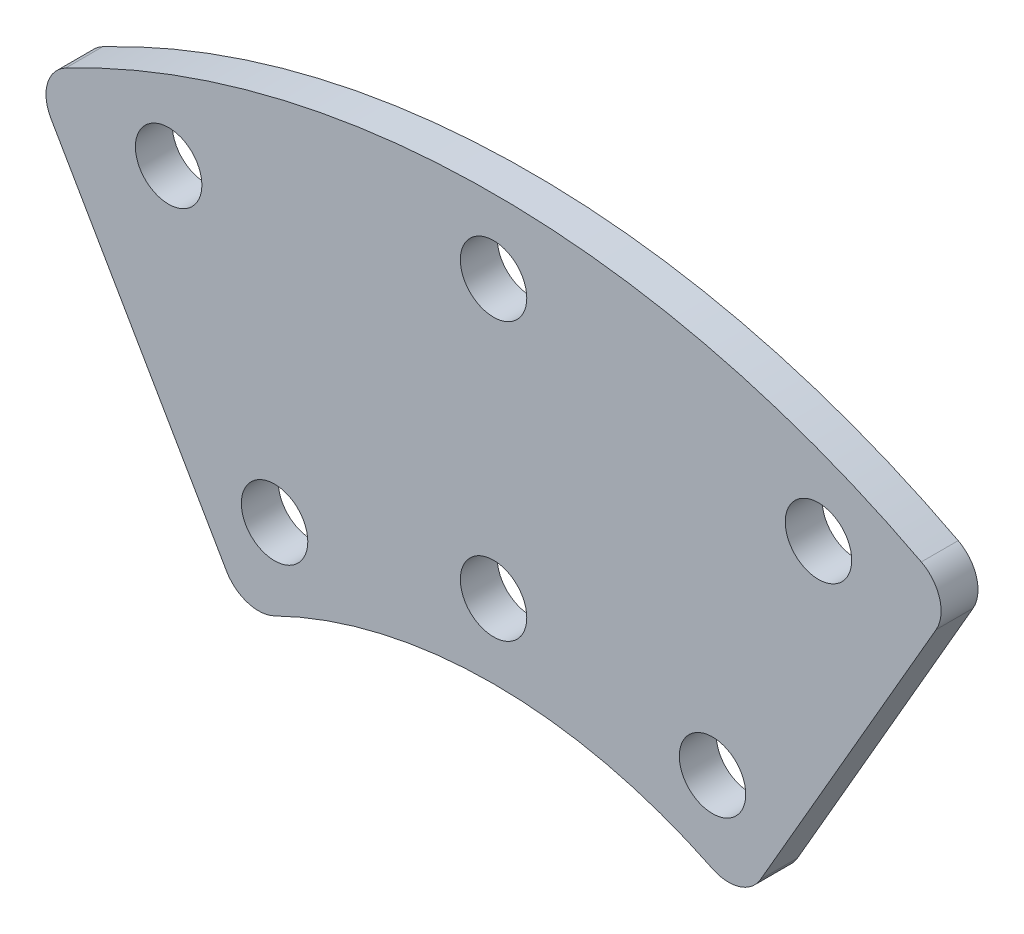
from build123d import *

# Parameters (mm, degrees)
SKETCH_1_R          = 9
EXTRUDE_1_DEPTH     = 10
FILLET_1_R          = 10
SKETCH_2_R          = 9
CUT_EXTRUDE_1_DEPTH = 279.025277116


with BuildPart() as part:
    # 草图1 → 凸台-拉伸1 (new body)
    with BuildSketch(Plane.XY):
        with BuildLine():
            Line((-67.5, 116.913429511), (-125, 216.506350946))
            ThreePointArc((-125, 216.506350946), (0, 250), (125, 216.506350946))
            Line((125, 216.506350946), (67.5, 116.913429511))
            ThreePointArc((67.5, 116.913429511), (0, 135), (-67.5, 116.913429511))
        make_face()
        with Locations((0, 155)):
            Circle(SKETCH_1_R, mode=Mode.SUBTRACT)
        with Locations((59.315932017, 143.201327539)):
            Circle(SKETCH_1_R, mode=Mode.SUBTRACT)
        with Locations((-59.315932017, 143.201327539)):
            Circle(SKETCH_1_R, mode=Mode.SUBTRACT)
    extrude(amount=EXTRUDE_1_DEPTH)

    # 圆角1
    fillet_1_edges = [part.edges().sort_by_distance(p)[0] for p in [
        (-67.5, 116.913429511, 5),
        (-125, 216.506350946, 5),
        (125, 216.506350946, 5),
        (67.5, 116.913429511, 5),
    ]]
    fillet(fillet_1_edges, radius=FILLET_1_R)

    # 草图2 → 切除-拉伸1 (cut, through all)
    with BuildSketch(Plane.XY.offset(10)):
        with Locations((0, 230)):
            Circle(SKETCH_2_R)
        with Locations((88.017189444, 212.492292478)):
            Circle(SKETCH_2_R)
        with Locations(Location((-88.017189444, 212.492292478, 0), (0, 0, 180))):
            Circle(SKETCH_2_R)
    extrude(amount=-CUT_EXTRUDE_1_DEPTH, mode=Mode.SUBTRACT)


solid = part.part
